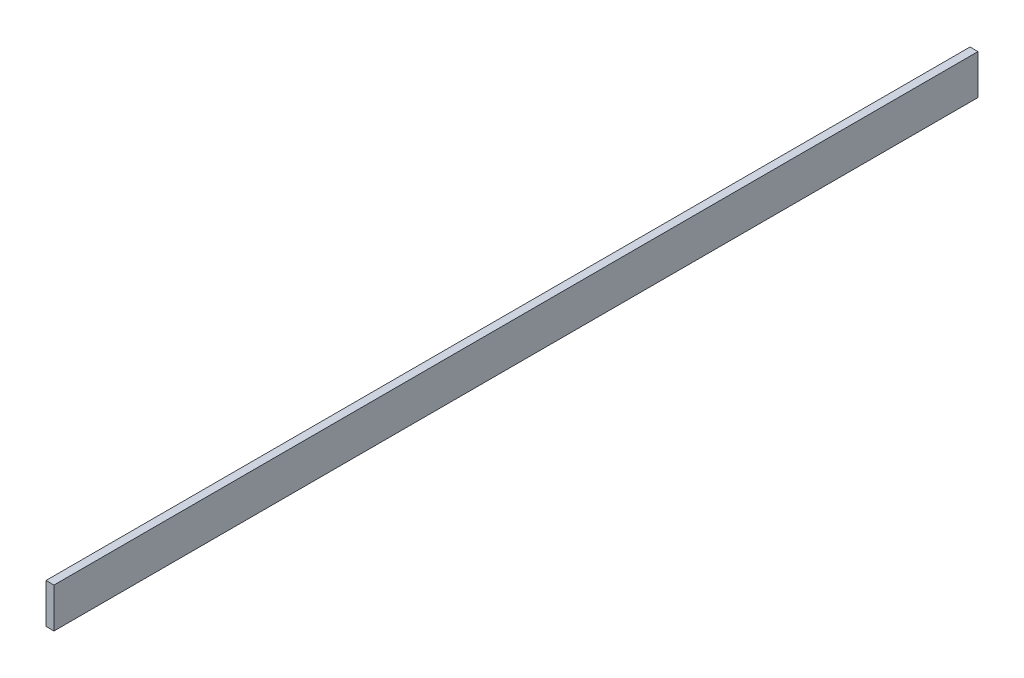
from build123d import *

# Parameters (mm, degrees)
SKETCH1_W           = 5
SKETCH1_H           = 25
BOSS_EXTRUDE1_DEPTH = 580


with BuildPart() as part:
    # Sketch1 → Boss-Extrude1 (new body)
    with BuildSketch(Plane.XY):
        with Locations((2.5, 12.5)):
            Rectangle(SKETCH1_W, SKETCH1_H)
    extrude(amount=BOSS_EXTRUDE1_DEPTH)


solid = part.part
